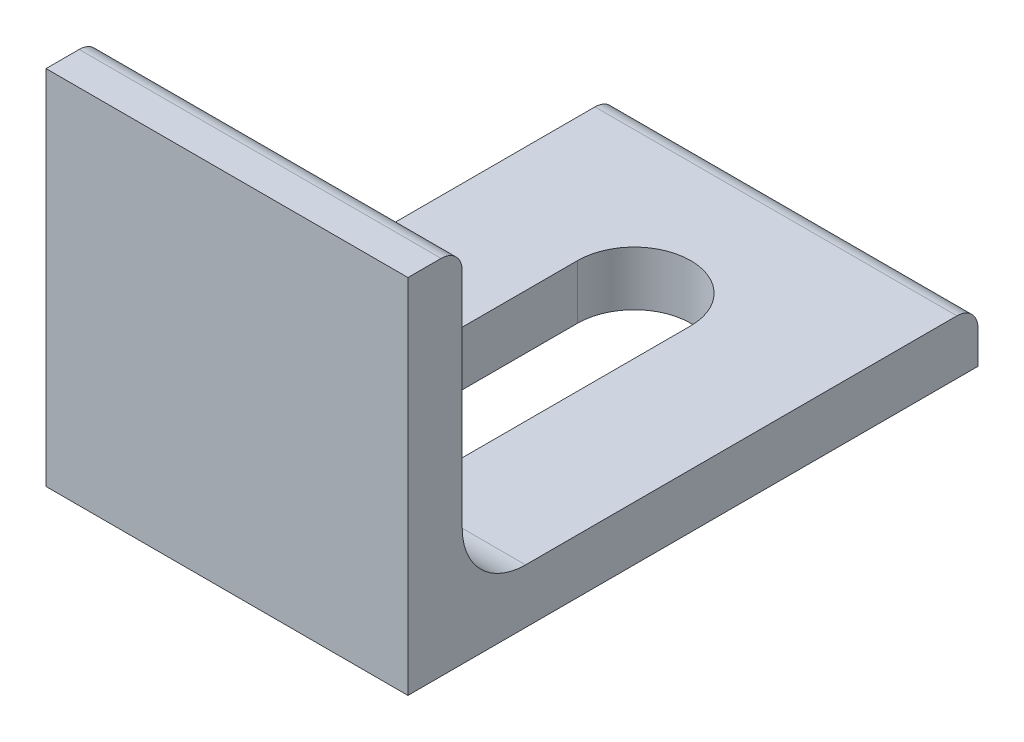
from build123d import *

# Parameters (mm, degrees)
GB_T706_2008_63_X_40_X_6_1_DEPTH = 40
CUT_EXTRUDE_1_DEPTH              = 10


with BuildPart() as part:
    # Sketch1 → 热轧不等边角钢gb∕t706-2008 63 X 40 X 6(1) (new body)
    with BuildSketch(Plane(origin=(220, 114, 0), x_dir=(0, 1, 0), z_dir=(-1, 0, 0))):
        with BuildLine():
            Line((0, 0), (0, 63))
            Line((0, 63), (3.666666667, 63))
            ThreePointArc((3.666666667, 63), (5.316582489, 62.316582489), (6, 60.666666667))
            Line((6, 60.666666667), (6, 13))
            ThreePointArc((6, 13), (8.050252532, 8.050252532), (13, 6))
            Line((13, 6), (37.666666667, 6))
            ThreePointArc((37.666666667, 6), (39.316582489, 5.316582489), (40, 3.666666667))
            Line((40, 3.666666667), (40, 0))
            Line((40, 0), (0, 0))
        make_face()
    extrude(amount=GB_T706_2008_63_X_40_X_6_1_DEPTH)

    # 草图2 → 切除-拉伸1 (cut)
    with BuildSketch(Plane(origin=(0, 120, 0), x_dir=(1, 0, 0), z_dir=(0, 1, 0))):
        with BuildLine():
            Line((206.25, 45), (206.25, 20))
            ThreePointArc((206.25, 20), (200, 13.75), (193.75, 20))
            Line((193.75, 20), (193.75, 45))
            ThreePointArc((193.75, 45), (200, 51.25), (206.25, 45))
        make_face()
    extrude(amount=-CUT_EXTRUDE_1_DEPTH, mode=Mode.SUBTRACT)


solid = part.part
